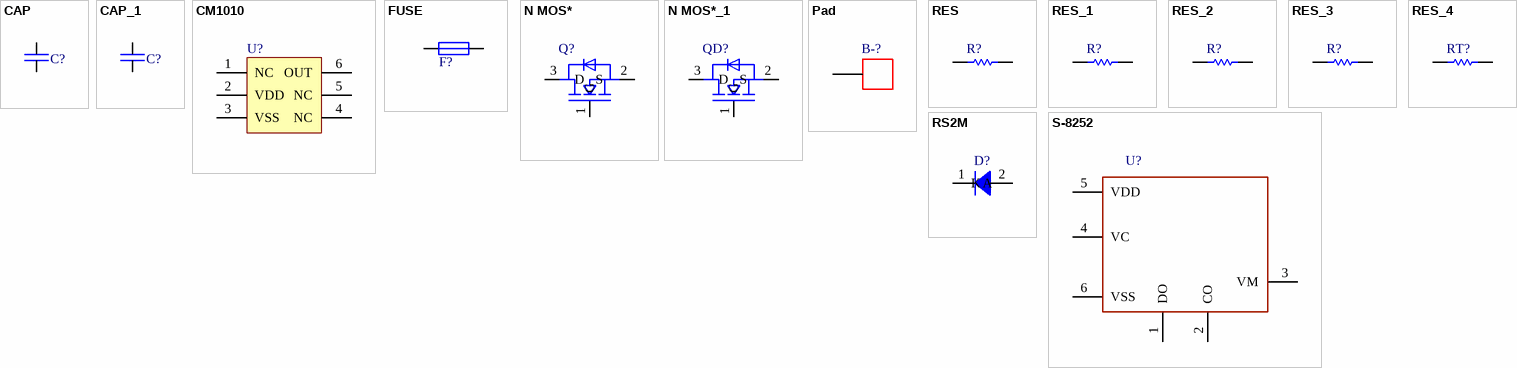
[diagram p0: symbols CAP to S-8252]
# Altium schematic symbol library MISC82045.SCHLIB: 14 symbols
Pins are listed as number, name and electrical type; pins without a type are passive.


## CAP
designator C?
SMD capacitor
footprint C0402A (SMD capacitor)
footprint C0603A (SMD capacitor)
footprint C0402L (SMD resistor)
footprint C0805A (SMD capacitor)
footprint C1206A (SMD capacitor)
footprint C0603L (SMD J-type capacitor)
footprint C0805L (SMD capacitor)
footprint C0603M (SMD capacitor)
footprint C0603A (SMD capacitor)
pins: 1, 2

## CAP_1
designator C?
SMD capacitor
footprint C0402A (SMD capacitor)
footprint C0603A (SMD capacitor)
footprint C0402L (SMD resistor)
footprint C0805A (SMD capacitor)
footprint C1206A (SMD capacitor)
footprint C0603L (SMD J-type capacitor)
footprint C0805L (SMD capacitor)
pins: 1, 2

## CM1010
designator U?
Chuangxinwei, balancing IC
footprint MSOP8
footprint SOT23-6A
pins: 1 NC, 2 VDD, 3 VSS, 4 NC, 5 NC, 6 OUT

## FUSE
designator F?
footprint R1206A (SMD resistor)
footprint R0603A (SMD resistor)
footprint R0805A (SMD resistor)
footprint F2410 (SMD fuse)
footprint J10*3mm (Jumper 10*3mm)
pins: 1, 2

## N MOS*
designator Q?
SMD MOSFET
footprint TO-252
footprint TO-252-DFN
footprint SOP-8L(T3p)
footprint DFN5X6(T3p) (SMD MOSFET (non-standard))
footprint TO-263-TOLL
footprint DFN-3x3L8(T3P) (SMD MOSFET)
footprint TOLL_123 (SMD MOSFET)
footprint TOLL_GSD (SMD MOSFET)
footprint SOT23-3L (SMD IMOS)
pins: 1 G, 2 S, 3 D

## N MOS*_1
designator QD?
SMD MOSFET
footprint TO-252
footprint TO-252-DFN
footprint DFN5X6(T3)
footprint SOP-8L(T3p)
footprint DFN5X6(T3p) (SMD MOSFET (non-standard))
footprint TO-263-TOLL
footprint DFN-3x3
footprint DFN-3x3L8(T3P) (SMD MOSFET)
footprint TOLL_123 (SMD MOSFET)
footprint TOLL_GSD (SMD MOSFET)
footprint TO-252
pins: 1 G, 2 S, 3 D

## Pad
designator B-?
Connection pad (non-through-hole)
footprint 3*3
footprint Pad10X8mm
footprint Pad8X6mm
pins: 1

## RES
designator R?
SMD resistor
footprint R0603A (SMD resistor)
footprint R0201A
footprint R0402A (SMD resistor)
footprint R0603m (SMD resistor)
footprint R0805A (SMD resistor)
footprint R0402L (SMD resistor)
footprint RES0603 (CAP0402)
footprint R0603L (SMD resistor)
footprint R0805L (SMD resistor)
footprint R0805M (SMD resistor)
footprint R1206A (SMD resistor)
pins: 1, 2

## RES_1
designator R?
SMD resistor
footprint R0603A (SMD resistor)
footprint R0201A
footprint R0402A (SMD resistor)
footprint R0603m (SMD resistor)
footprint R0805A (SMD resistor)
footprint R0402L (SMD resistor)
footprint RES0603 (CAP0402)
footprint R0603L (SMD resistor)
footprint R0805L (SMD resistor)
footprint R0805M (SMD resistor)
footprint R1206A (SMD resistor)
pins: 1, 2

## RES_2
designator R?
SMD resistor
footprint R0603A (SMD resistor)
footprint R0201A
footprint R0402A (SMD resistor)
footprint R0603m (SMD resistor)
footprint R0805A (SMD resistor)
footprint R0402L (SMD resistor)
footprint RES0603 (CAP0402)
footprint R0603L (SMD resistor)
footprint R0805L (SMD resistor)
pins: 1, 2

## RES_3
designator R?
SMD resistor
footprint R0603A (SMD resistor)
footprint R0201A
footprint R0402A (SMD resistor)
footprint R0603m (SMD resistor)
footprint R0805A (SMD resistor)
footprint R0402L (SMD resistor)
footprint RES0603 (CAP0402)
footprint R0603L (SMD resistor)
footprint R0805L (SMD resistor)
pins: 1, 2

## RES_4
designator RT?
SMD resistor
footprint R0603A (SMD resistor)
footprint R0201A
footprint R0402A (SMD resistor)
footprint R0603m (SMD resistor)
footprint R0805A (SMD resistor)
footprint R0402L (SMD resistor)
footprint RES0603 (CAP0402)
footprint R0603L (SMD resistor)
footprint R0805L (SMD resistor)
pins: 1, 2

## RS2M
designator D?
SMD diode
footprint SMA(DO-214AC) (SMD diode)
footprint SMB(DO-214AA) (SMD diode)
footprint SMB A (1+2-) (SMD diode)
pins: 1 A, 2 K

## S-8252
designator U?
2S battery protection IC
footprint SOT23-6A
footprint SOT23-6M (SMD MOSFET (special application)!!!)
pins: 1 DO, 2 CO, 3 VM, 4 VC, 5 VDD, 6 VSS